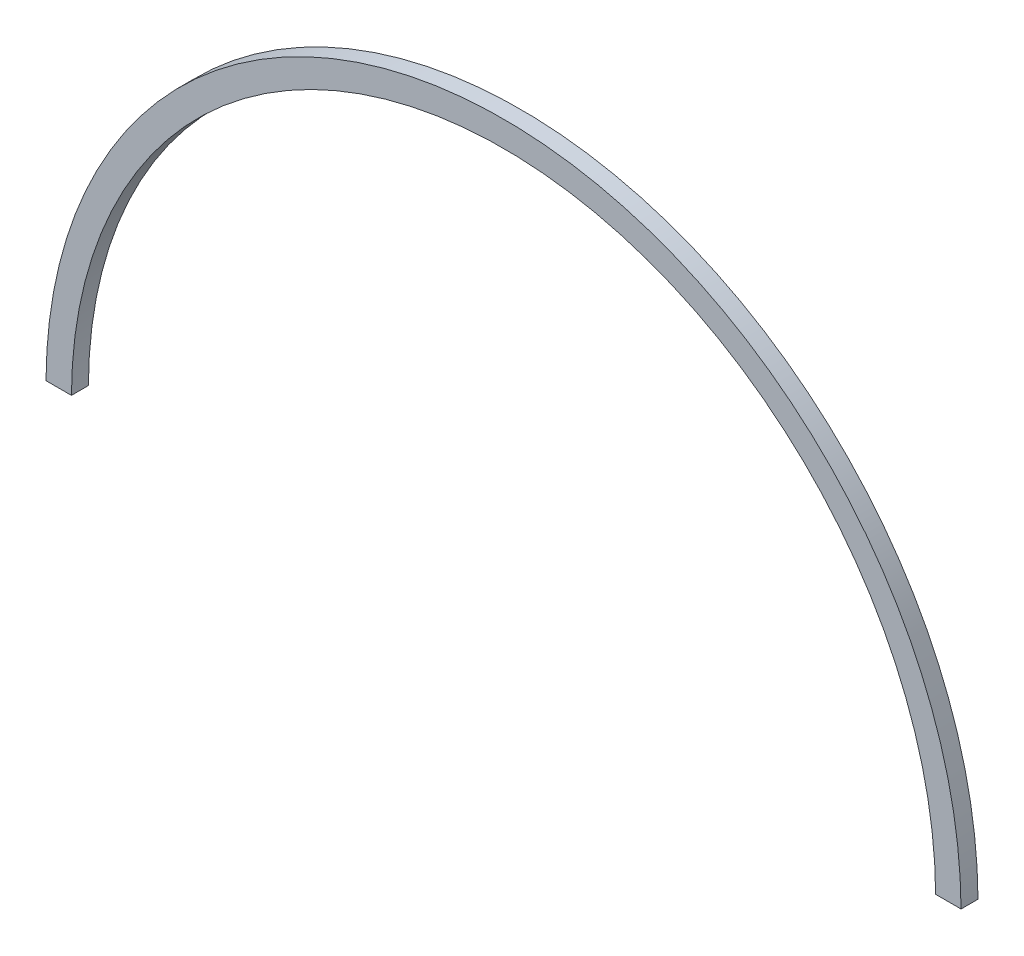
SolidWorks part; units mm, degrees
ref_plane "前视基准面" through (0, 0, 0) normal (0, 0, 1) x (1, 0, 0)
ref_plane "上视基准面" through (0, 0, 0) normal (0, 1, 0) x (1, 0, 0)
ref_plane "右视基准面" through (0, 0, 0) normal (1, 0, 0) x (0, 0, -1)
other "Configuration Table"
sketch "草图1" plane through (0, 0, 0) normal (0, 0, 1) x (1, 0, 0)
  line L0 (4.0023, 1) -> (16.0025, 1)
  line L1 (423.9975, 1) -> (435.9977, 1)
  arc A0 (435.9977, 1) -> (4.0023, 1) centre (220, 0) ccw
  arc A1 (16.0025, 1) -> (423.9975, 1) centre (220, 0) cw
  point P0 (0, 0)
  dimension "D1" = 216
  dimension "D2" = 204
  dimension "D3" = 12.0001
  dimension "D4" = 435.9977
extrude "凸台-拉伸1" add sketch "草图1" against normal mid plane 8
